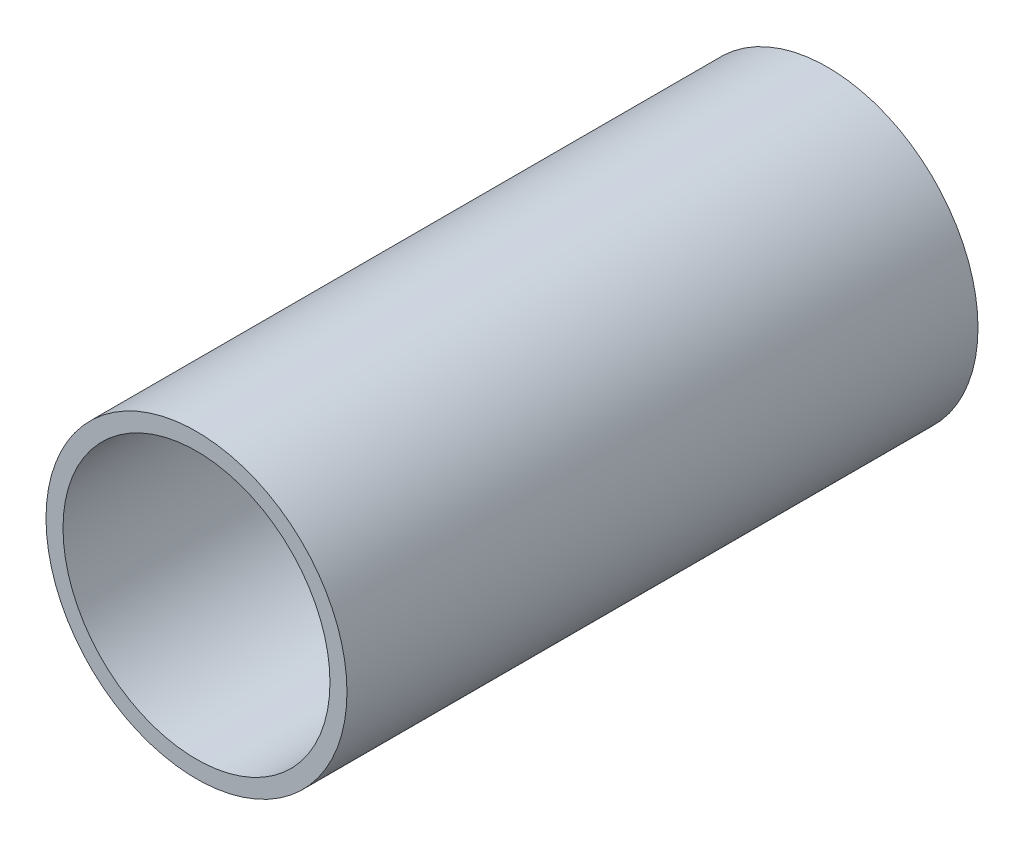
from build123d import *

# Parameters (mm, degrees)
SKETCH_1_R      = 31
SKETCH_1_R_2    = 27.5
EXTRUDE_1_DEPTH = 130


with BuildPart() as part:
    # 草图1 → 凸台-拉伸1 (new body)
    with BuildSketch(Plane.XY):
        Circle(SKETCH_1_R)
        Circle(SKETCH_1_R_2, mode=Mode.SUBTRACT)
    extrude(amount=EXTRUDE_1_DEPTH)


solid = part.part
